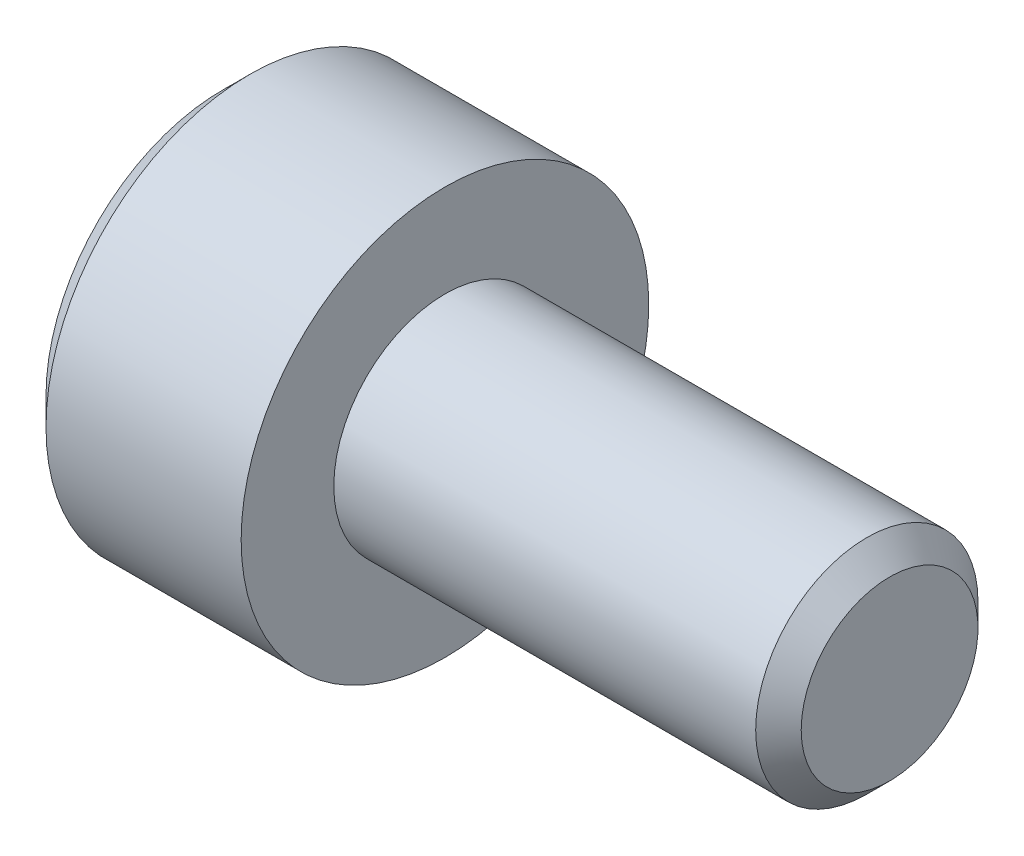
from build123d import *

# Parameters (mm, degrees)
CUT_EXTRUDE1_DEPTH = 1.5


with BuildPart() as part:
    # Sketch1 → Revolve1 (revolve)
    with BuildSketch(Plane.XY, mode=Mode.PRIVATE) as revolve1_sk:
        Polygon((-3, 0), (-3, 2.383333333), (-2.633333333, 2.75), (0, 2.75), (0, 1.5), (5.6928325, 1.5), (6, 1.1928325), (6, 0), align=None)
    revolve(revolve1_sk.sketch.rotate(Axis((6, 0, 0), (-1, 0, 0)), 270), axis=Axis((6, 0, 0), (-1, 0, 0)))

    # Sketch2 → Cut-Revolve1 (revolve, cut)
    with BuildSketch(Plane.XY, mode=Mode.PRIVATE) as cut_revolve1_sk:
        Polygon((-3, 0), (-3, 1.25), (-1.5, 1.25), (-1.165063509, 0), align=None)
    revolve(cut_revolve1_sk.sketch.rotate(Axis((-1.165063509, 0, 0), (-1, 0, 0)), 270), axis=Axis((-1.165063509, 0, 0), (-1, 0, 0)), mode=Mode.SUBTRACT)

    # Sketch3 → Cut-Extrude1 (cut)
    with BuildSketch(Plane(origin=(-3, 0, 0), x_dir=(0, 0, -1), z_dir=(1, 0, 0))):
        Polygon((-1.25, 0.721687836), (-1.25, -0.721687836), (0, -1.443375673), (1.25, -0.721687836), (1.25, 0.721687836), (0, 1.443375673), align=None)
    extrude(amount=CUT_EXTRUDE1_DEPTH, mode=Mode.SUBTRACT)


solid = part.part
